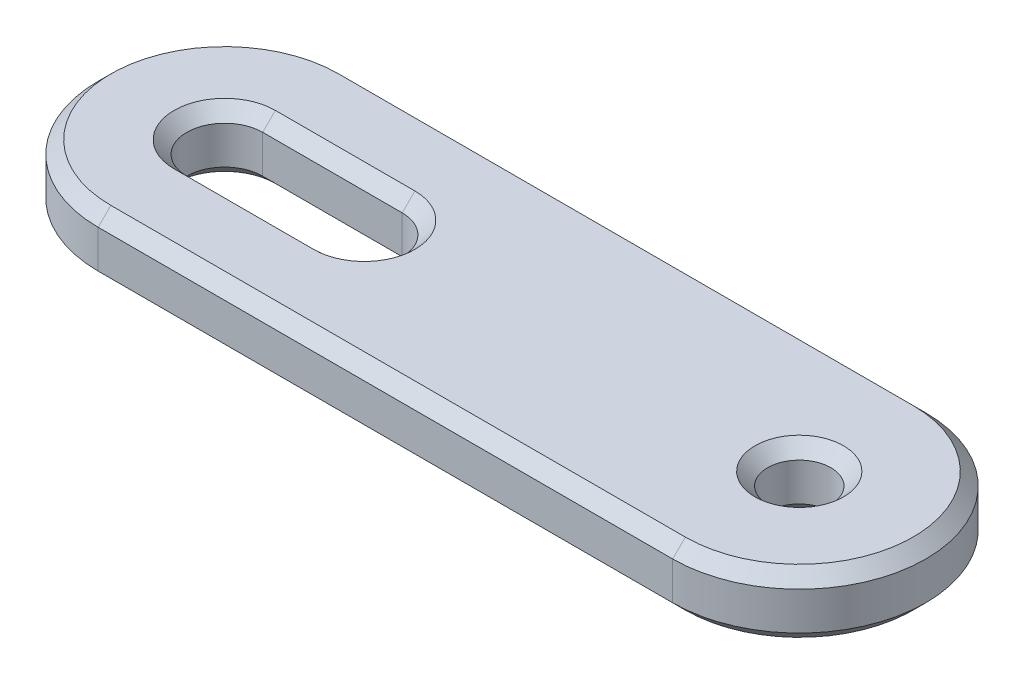
SolidWorks part; units mm, degrees
ref_plane "Front Plane" through (0, 0, 0) normal (0, 0, 1) x (1, 0, 0)
ref_plane "Top Plane" through (0, 0, 0) normal (0, 1, 0) x (1, 0, 0)
ref_plane "Right Plane" through (0, 0, 0) normal (1, 0, 0) x (0, 0, -1)
other "Configuration Table"
sketch "Sketch1" plane through (0, 0, 0) normal (0, 1, 0) x (1, 0, 0)
  line L0 (0, 0) -> (-45.3981, 0) construction
  line L1 (0, -10) -> (-45.3981, -10)
  line L2 (0, 10) -> (-45.3981, 10)
  line L3 (-45.3981, 0) -> (-34.3728, 0) construction
  line L4 (-45.3981, 3) -> (-34.3728, 3)
  line L5 (-45.3981, -3) -> (-34.3728, -3)
  arc A0 (0, -10) -> (0, 10) centre (0, 0) ccw
  arc A1 (-45.3981, 10) -> (-45.3981, -10) centre (-45.3981, 0) ccw
  circle A2 centre (0, 0) radius 2.5
  arc A3 (-45.3981, 3) -> (-45.3981, -3) centre (-45.3981, 0) ccw
  arc A4 (-34.3728, -3) -> (-34.3728, 3) centre (-34.3728, 0) ccw
  point P3 (-22.699, 0)
  point P12 (-39.8854, 0)
  dimension "D1" = 5
  dimension "D2" = 10
  dimension "D3" = 3
extrude "Boss-Extrude1" add sketch "Sketch1" along normal blind 5
chamfer "Chamfer1" distance 1 angle 45 18 edges at (-39.8854, 0, -3) (-31.3728, 0, 0) (-39.8854, 0, 3) (-48.3981, 0, 0) (-22.699, 0, -10) (-55.3981, 0, 0) (-22.699, 0, 10) (10, 0, 0) (0, 0, 2.5) (-31.3728, 5, 0) (-39.8854, 5, -3) (-48.3981, 5, 0) (-39.8854, 5, 3) (0, 5, 2.5) (-22.699, 5, 10) (-55.3981, 5, 0) (-22.699, 5, -10) (10, 5, 0)
